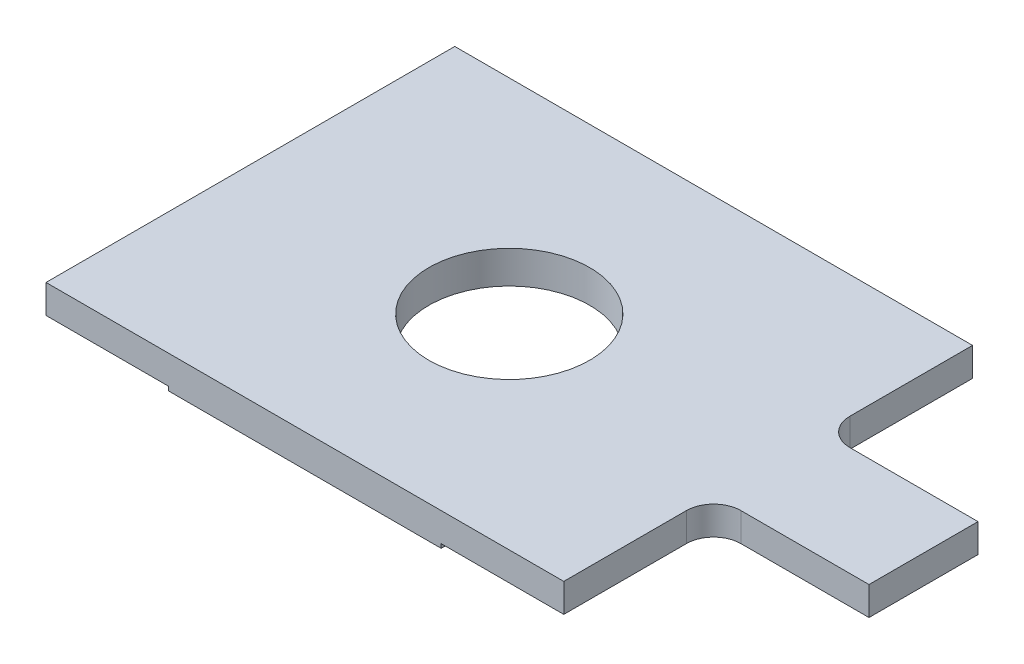
from build123d import *

# Parameters (mm, degrees)
EXTRUDE_1_DEPTH     = 75
CUT_EXTRUDE_1_REACH = 123.631
SKETCH_2_R          = 29.5
SKETCH_4_W          = 40
SKETCH_4_H          = 10.5
EXTRUDE_2_DEPTH     = 57
FILLET_1_R          = 10


with BuildPart() as part:
    # 草图1 → 凸台-拉伸1 (new, symmetric)
    with BuildSketch(Plane.XY):
        Polygon((0, 0), (-50, 0), (-50, 1.5), (-95, 1.5), (-95, 12), (95, 12), (95, 1.5), (50, 1.5), (50, 0), align=None)
    extrude(amount=EXTRUDE_1_DEPTH, both=True)

    # 草图2 → 切除-拉伸1 (cut, up to next)
    with BuildSketch(Plane(origin=(0, 12, 0), x_dir=(1, 0, 0), z_dir=(0, 1, 0)), mode=Mode.PRIVATE) as cut_extrude_1_sk1:
        with Locations(Location((0, 0, 0), (0, 0, 270))):
            Circle(SKETCH_2_R)
    cut_extrude_1_tool1 = extrude(cut_extrude_1_sk1.sketch, amount=-CUT_EXTRUDE_1_REACH, mode=Mode.PRIVATE) & part.part
    add(cut_extrude_1_tool1.solids().sort_by_distance((0, 12, 0))[0], mode=Mode.SUBTRACT)

    # 草图4 → 凸台-拉伸2 (add)
    with BuildSketch(Plane(origin=(95, 0, 0), x_dir=(0, 0, -1), z_dir=(1, 0, 0))):
        with Locations((0, 6.75)):
            Rectangle(SKETCH_4_W, SKETCH_4_H)
    extrude(amount=EXTRUDE_2_DEPTH)

    # 圆角1
    fillet_1_edges = [part.edges().sort_by_distance(p)[0] for p in [
        (95, 6.75, 20),
        (95, 6.75, -20),
    ]]
    fillet(fillet_1_edges, radius=FILLET_1_R)


solid = part.part
